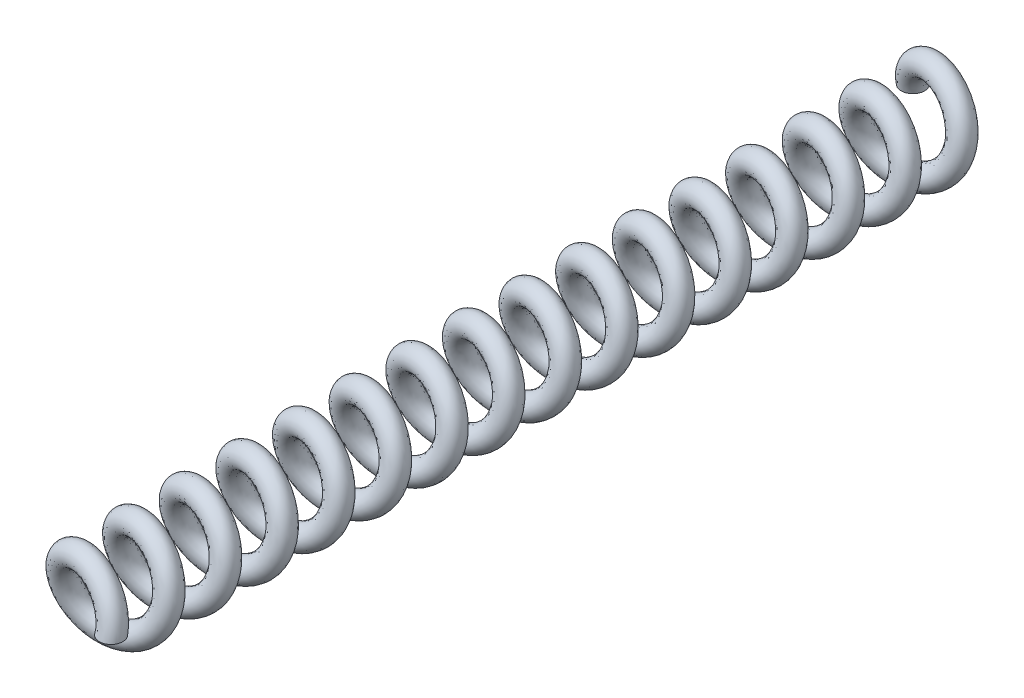
from build123d import *

# Parameters (mm, degrees)
SWEEP_1_PITCH       = 9.677419355
SWEEP_1_HEIGHT      = 150
SWEEP_1_RADIUS      = 6.5
SWEEP_1_START_ANGLE = -180
SKETCH_2_R          = 2


with BuildPart() as part:
    # 扫描1: sweep along a helix
    with BuildLine() as sweep_1_path:
        add(Helix(SWEEP_1_PITCH, SWEEP_1_HEIGHT, SWEEP_1_RADIUS, center=(0, 0, 0), direction=(0, 0, 1), lefthand=True, mode=Mode.PRIVATE).rotate(Axis((0, 0, 0), (0, 0, 1)), SWEEP_1_START_ANGLE))
    # 草图2 → 扫描1 (sweep)
    with BuildSketch(Plane(origin=(0, 0, 0), x_dir=(1, 0, 0), z_dir=(0, 1, 0))):
        with Locations((-6.5, 0)):
            Circle(SKETCH_2_R)
    sweep(path=sweep_1_path.line, is_frenet=True)


solid = part.part
